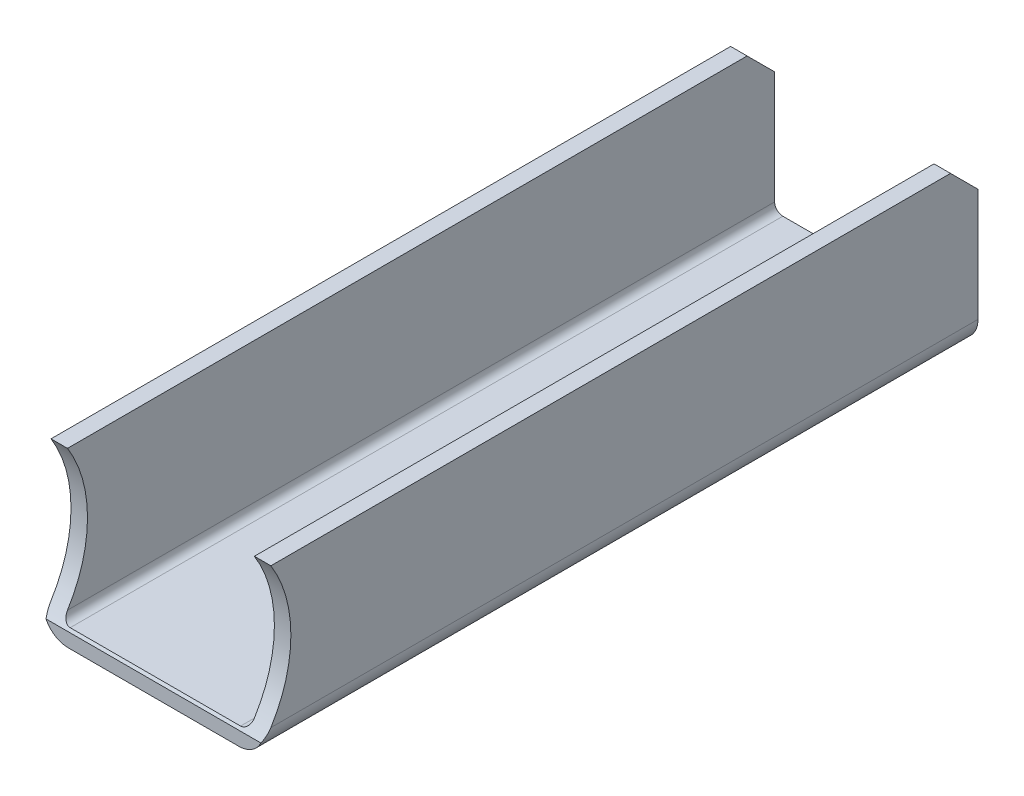
SolidWorks part; units mm, degrees
material "1023 碳钢板 (SS)"
ref_plane "Front Plane" through (0, 0, 0) normal (0, 0, 1) x (1, 0, 0)
ref_plane "Top Plane" through (0, 0, 0) normal (0, 1, 0) x (1, 0, 0)
ref_plane "Right Plane" through (0, 0, 0) normal (1, 0, 0) x (0, 0, -1)
sketch "Sketch1" plane through (0, 0, 0) normal (0, 0, 1) x (1, 0, 0)
  line L0 (0, 0) -> (0, -25.5)
  line L1 (4.5, -30) -> (35.5, -30)
  line L2 (40, -25.5) -> (40, 0)
  line L3 (3, 0) -> (3, -25.5)
  line L4 (4.5, -27) -> (35.5, -27)
  line L5 (37, -25.5) -> (37, 0)
  line L6 (3, 0) -> (0, 0)
  line L7 (37, 0) -> (40, 0)
  arc A0 (35.5, -30) -> (40, -25.5) centre (35.5, -25.5) ccw
  arc A1 (0, -25.5) -> (4.5, -30) centre (4.5, -25.5) ccw
  arc A2 (3, -25.5) -> (4.5, -27) centre (4.5, -25.5) ccw
  arc A3 (35.5, -27) -> (37, -25.5) centre (35.5, -25.5) ccw
  point P7 (40, -30)
  point P10 (0, -30)
  dimension "D4" = 4.5
  dimension "D1" = 30
  dimension "D2" = 30
  dimension "D3" = 40
  dimension "D5" = 3
extrude "Boss-Extrude1" add sketch "Sketch1" along normal blind 130
chamfer "Chamfer1" distance 5 angle 45 2 edges at (1.5, 0, 0) (38.5, 0, 0)
sketch "Sketch2" plane through (40, 0, 0) normal (1, 0, 0) x (0, 0, -1)
  line L2 (-130, -25.5) -> (-130, 0) construction
  line L3 (0, -25.5) -> (0, -5) construction
  circle A0 centre (-149.15, -12.75) radius 24.15
  point P7 (-130, -12.75)
  dimension "D1" = 48.3
  dimension "D2" = 149.15
extrude "Cut-Extrude1" cut sketch "Sketch2" against normal blind 130
sketch "Sketch3" plane through (0, -30, 0) normal (0, -1, 0) x (1, 0, 0)
  line L0 (20, 96) -> (20, 21) construction
  line L1 (24.5, 96) -> (24.5, 21)
  line L2 (15.5, 96) -> (15.5, 21)
  line L3 (4.5, 0) -> (35.5, 0) construction
  arc A0 (24.5, 96) -> (15.5, 96) centre (20, 96) ccw
  arc A1 (15.5, 21) -> (24.5, 21) centre (20, 21) ccw
  point P2 (20, 58.5)
  point P10 (20, 0)
  dimension "D3" = 4.5
  dimension "D1" = 21
  dimension "D2" = 75
extrude "Cut-Extrude2" cut sketch "Sketch3" against normal blind 130
